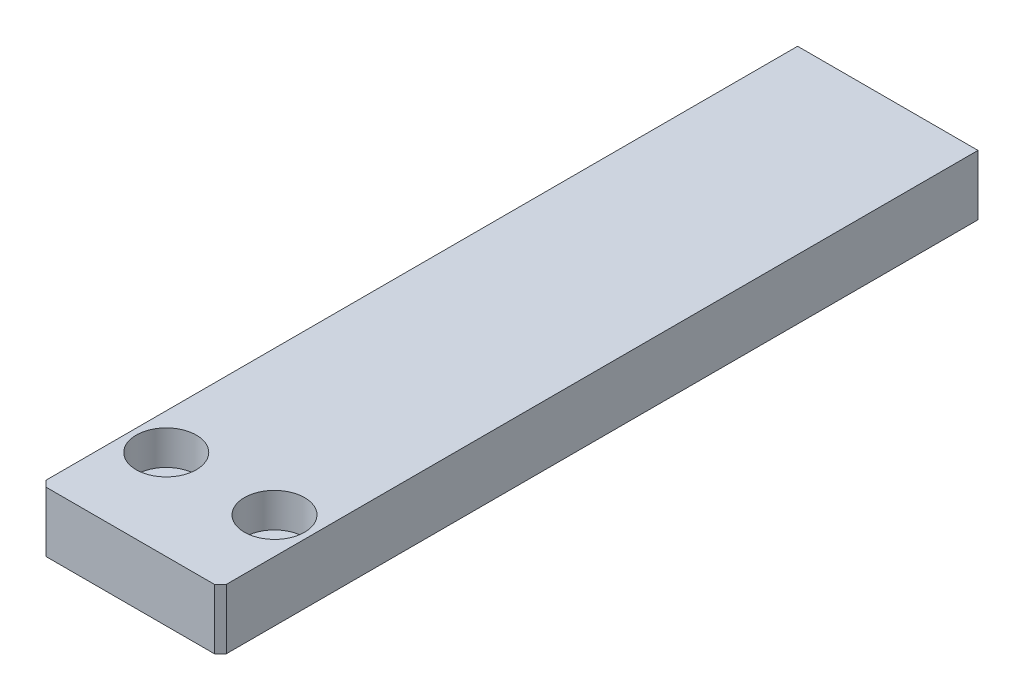
from build123d import *

# Parameters (mm, degrees)
SKETCH_1_W                = 30
SKETCH_1_H                = 126
EXTRUDE_1_DEPTH           = 5
HOLE_WIZARD_1_D           = 5.5
HOLE_WIZARD_1_CBORE_D     = 10
HOLE_WIZARD_1_CBORE_DEPTH = 5.7
CHAMFER_1_SIZE            = 1
HOLE_WIZARD_M4_1_D        = 3.3
HOLE_WIZARD_M4_1_DEPTH    = 10.1
HOLE_WIZARD_M4_1_TIP      = 0.991420021


with BuildPart() as part:
    # 草图1 → 凸台-拉伸1 (new, symmetric)
    with BuildSketch(Plane(origin=(0, 0, 0), x_dir=(1, 0, 0), z_dir=(0, 1, 0))):
        Rectangle(SKETCH_1_W, SKETCH_1_H)
    extrude(amount=EXTRUDE_1_DEPTH, both=True)

    # 打孔尺寸(%根据)内六角圆柱头螺钉的类型1 (through all)
    with Locations(Plane(origin=(0, 5, 0), x_dir=(1, 0, 0), z_dir=(0, 1, 0))):
        with Locations((9, -48), (-9, -48)):
            CounterBoreHole(HOLE_WIZARD_1_D / 2, HOLE_WIZARD_1_CBORE_D / 2, HOLE_WIZARD_1_CBORE_DEPTH)

    # 倒角1
    chamfer_1_edges = [part.edges().sort_by_distance(p)[0] for p in [
        (15, 0, 63),
        (-15, 0, 63),
    ]]
    chamfer(chamfer_1_edges, length=CHAMFER_1_SIZE)

    # M4 螺纹孔1
    with Locations(Plane(origin=(0, 0, -63), x_dir=(-1, 0, 0), z_dir=(0, 0, -1))):
        with Locations((-10, 0), (10, 0)):
            Hole(HOLE_WIZARD_M4_1_D / 2, depth=HOLE_WIZARD_M4_1_DEPTH)
            with Locations((0, 0, -(HOLE_WIZARD_M4_1_DEPTH + HOLE_WIZARD_M4_1_TIP / 2))):  # 118° drill point
                Cone(0, HOLE_WIZARD_M4_1_D / 2, HOLE_WIZARD_M4_1_TIP, mode=Mode.SUBTRACT)


solid = part.part
